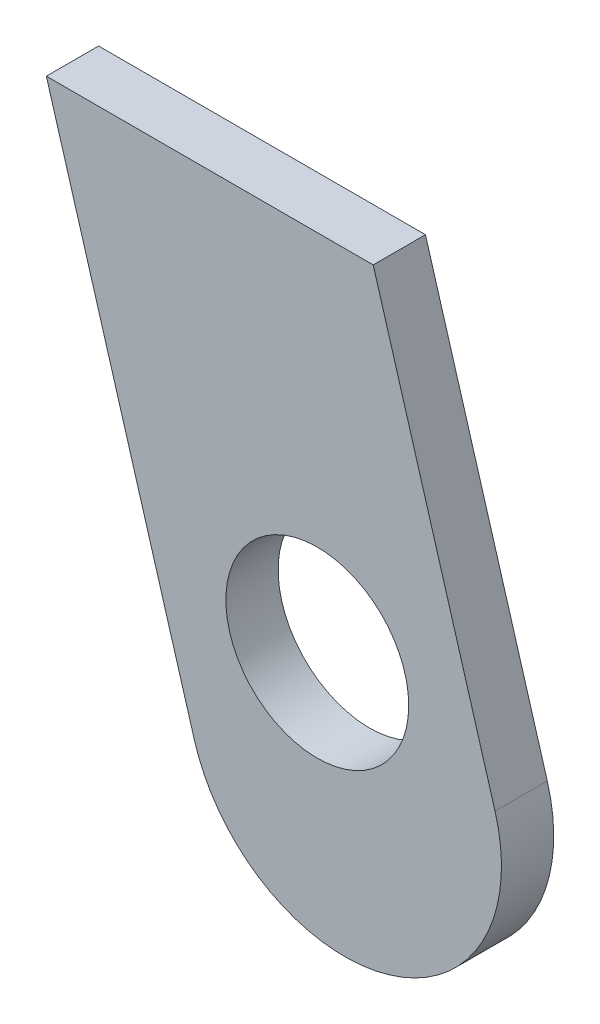
SolidWorks part; units mm, degrees
ref_plane "前视基准面" through (0, 0, 0) normal (0, 0, 1) x (1, 0, 0)
ref_plane "上视基准面" through (0, 0, 0) normal (0, 1, 0) x (1, 0, 0)
ref_plane "右视基准面" through (0, 0, 0) normal (1, 0, 0) x (0, 0, -1)
sketch "草图2" plane through (0, 0, 0) normal (0, 0, 1) x (1, 0, 0)
  line L0 (507.0654, -222.1227) -> (535.4093, -318.0217)
  line L1 (-900.6034, -222.1227) -> (1399.1334, -222.1227) construction
  line L2 (569.6312, -222.1227) -> (592.9487, -301.0154)
  line L3 (507.0654, -222.1227) -> (569.6312, -222.1227)
  line L4 (564.6048, -205.1163) -> (592.9487, -301.0154) construction
  circle A0 centre (558.9278, -291.7515) radius 17.5
  arc A1 (535.4093, -318.0217) -> (592.9487, -301.0154) centre (564.179, -309.5185) ccw
  circle A2 centre (558.9278, -291.7515) radius 12 construction
  dimension "D3" = 35
  dimension "D2" = 30
  dimension "D4" = 100
  dimension "D1" = 60
extrude "凸台-拉伸1" add sketch "草图2" against normal blind 10
